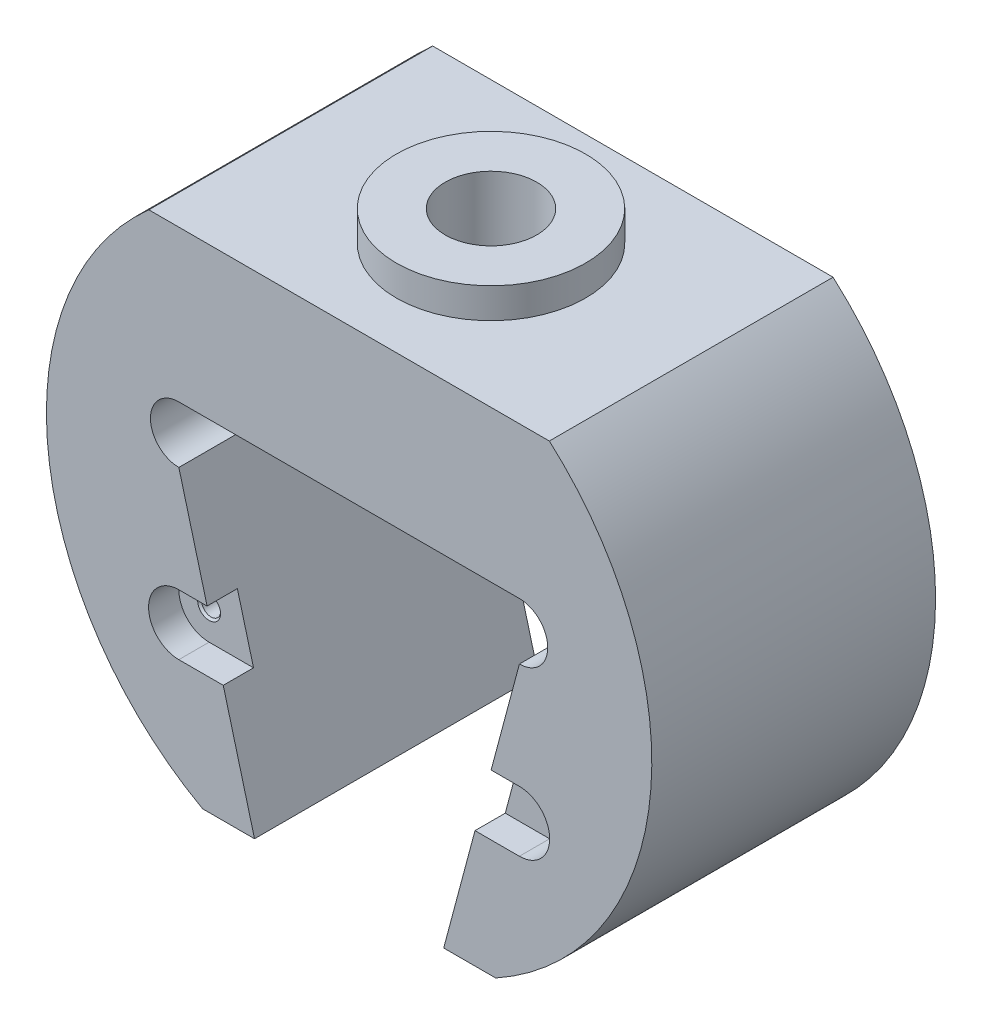
from build123d import *

# Parameters (mm, degrees)
SKETCH1_R                             = 80
BOSS_EXTRUDE1_DEPTH                   = 75
SKETCH2_OUTSIDE_W                     = 209.676
SKETCH2_OUTSIDE_H                     = 209.676
SKETCH2_OUTSIDE_W_2                   = 199.64377861
SKETCH2_OUTSIDE_H_2                   = 130
CUT_EXTRUDE1_DEPTH                    = 136.738719605
CUT_EXTRUDE2_DEPTH                    = 131.096118313
CUT_EXTRUDE3_DEPTH                    = 8
CUT_EXTRUDE4_START                    = -59
CUT_EXTRUDE4_DEPTH                    = 8
M6_TAPPED_HOLE1_D                     = 5
M6_TAPPED_HOLE1_DEPTH                 = 15
M6_TAPPED_HOLE1_CSINK_D               = 6.05
M6_TAPPED_HOLE1_CSINK_ANGLE           = 90
M6_TAPPED_HOLE1_TIP                   = 1.502151548
M6_TAPPED_HOLE1_ON_FACE_2_D           = 5
M6_TAPPED_HOLE1_ON_FACE_2_DEPTH       = 15
M6_TAPPED_HOLE1_ON_FACE_2_CSINK_D     = 6.05
M6_TAPPED_HOLE1_ON_FACE_2_CSINK_ANGLE = 90
M6_TAPPED_HOLE1_ON_FACE_2_TIP         = 1.502151548
CUT_EXTRUDE5_REACH                    = 172.074
SKETCH7_R                             = 12.1
BOSS_EXTRUDE4_START                   = 8
SKETCH8_R                             = 25
SKETCH8_R_2                           = 12.1
BOSS_EXTRUDE4_DEPTH                   = 8


with BuildPart() as part:
    # Sketch1 → Boss-Extrude1 (new body)
    with BuildSketch(Plane.XY):
        Circle(SKETCH1_R)
    extrude(amount=BOSS_EXTRUDE1_DEPTH)

    # Sketch2 outside → Cut-Extrude1 (cut, through all)
    with BuildSketch(Plane(origin=(0, 0, 0), x_dir=(-1, 0, 0), z_dir=(0, 0, -1))):
        Rectangle(SKETCH2_OUTSIDE_W, SKETCH2_OUTSIDE_H)
        with Locations((0.958801498, -5)):
            Rectangle(SKETCH2_OUTSIDE_W_2, SKETCH2_OUTSIDE_H_2, mode=Mode.SUBTRACT)
    extrude(amount=-CUT_EXTRUDE1_DEPTH, mode=Mode.SUBTRACT)

    # Sketch3 → Cut-Extrude2 (cut, through all)
    with BuildSketch(Plane(origin=(0, 0, 0), x_dir=(-1, 0, 0), z_dir=(0, 0, -1))):
        with BuildLine():
            Line((-25, -70), (-45, 5))
            ThreePointArc((-45, 5), (-52.5, 12.5), (-45, 20))
            Line((-45, 20), (45, 20))
            ThreePointArc((45, 20), (52.5, 12.5), (45, 5))
            Line((45, 5), (25, -70))
            Line((25, -70), (-25, -70))
        make_face()
    extrude(amount=-CUT_EXTRUDE2_DEPTH, mode=Mode.SUBTRACT)

    # Sketch4 → Cut-Extrude3 (cut)
    with BuildSketch(Plane(origin=(0, 0, 0), x_dir=(-1, 0, 0), z_dir=(0, 0, -1))):
        with BuildLine():
            Line((-45, -23), (45, -23))
            ThreePointArc((45, -23), (53, -31), (45, -39))
            Line((45, -39), (-45, -39))
            ThreePointArc((-45, -39), (-53, -31), (-45, -23))
        make_face()
    extrude(amount=-CUT_EXTRUDE3_DEPTH, mode=Mode.SUBTRACT)

    # Sketch5 → Cut-Extrude4 (cut)
    with BuildSketch(Plane(origin=(0, 0, 8), x_dir=(-1, 0, 0), z_dir=(0, 0, -1)).offset(CUT_EXTRUDE4_START)):
        with BuildLine():
            Line((37.533333333, -23), (33.266666667, -39))
            Line((33.266666667, -39), (45, -39))
            ThreePointArc((45, -39), (53, -31), (45, -23))
            Line((45, -23), (37.533333333, -23))
        make_face()
        with BuildLine():
            Line((-33.266666667, -39), (-37.533333333, -23))
            Line((-37.533333333, -23), (-45, -23))
            ThreePointArc((-45, -23), (-53, -31), (-45, -39))
            Line((-45, -39), (-33.266666667, -39))
        make_face()
    extrude(amount=-CUT_EXTRUDE4_DEPTH, mode=Mode.SUBTRACT)

    # M6 Tapped Hole1
    with Locations(Plane(origin=(45, -31, 8), x_dir=(-1, 0, 0), z_dir=(0, 0, -1))):
        with Locations((0, 0), (90, 0)):
            CounterSinkHole(M6_TAPPED_HOLE1_D / 2, M6_TAPPED_HOLE1_CSINK_D / 2, depth=M6_TAPPED_HOLE1_DEPTH, counter_sink_angle=M6_TAPPED_HOLE1_CSINK_ANGLE)
            with Locations((0, 0, -(M6_TAPPED_HOLE1_DEPTH + M6_TAPPED_HOLE1_TIP / 2))):  # 118° drill point
                Cone(0, M6_TAPPED_HOLE1_D / 2, M6_TAPPED_HOLE1_TIP, mode=Mode.SUBTRACT)

    # M6 Tapped Hole1 on face 2
    with Locations(Plane(origin=(-45, -31, 67), x_dir=(1, 0, 0), z_dir=(0, 0, 1))):
        with Locations((0, 0), (90, 0)):
            CounterSinkHole(M6_TAPPED_HOLE1_ON_FACE_2_D / 2, M6_TAPPED_HOLE1_ON_FACE_2_CSINK_D / 2, depth=M6_TAPPED_HOLE1_ON_FACE_2_DEPTH, counter_sink_angle=M6_TAPPED_HOLE1_ON_FACE_2_CSINK_ANGLE)
            with Locations((0, 0, -(M6_TAPPED_HOLE1_ON_FACE_2_DEPTH + M6_TAPPED_HOLE1_ON_FACE_2_TIP / 2))):  # 118° drill point
                Cone(0, M6_TAPPED_HOLE1_ON_FACE_2_D / 2, M6_TAPPED_HOLE1_ON_FACE_2_TIP, mode=Mode.SUBTRACT)

    # Sketch7 → Cut-Extrude5 (cut, up to next)
    with BuildSketch(Plane(origin=(0, 60, 0), x_dir=(1, 0, 0), z_dir=(0, 1, 0)), mode=Mode.PRIVATE) as cut_extrude5_sk1:
        with Locations(Location((0, -37.5, 0), (0, 0, 270))):
            Circle(SKETCH7_R)
    cut_extrude5_tool1 = extrude(cut_extrude5_sk1.sketch, amount=-CUT_EXTRUDE5_REACH, mode=Mode.PRIVATE) & part.part
    add(cut_extrude5_tool1.solids().sort_by_distance((0, 60, 37.5))[0], mode=Mode.SUBTRACT)

    # Sketch8 → Boss-Extrude4 (add)
    with BuildSketch(Plane(origin=(0, 60, 0), x_dir=(1, 0, 0), z_dir=(0, 1, 0)).offset(BOSS_EXTRUDE4_START)):
        with Locations(Location((0, -37.5, 0), (0, 0, 270))):
            Circle(SKETCH8_R)
        with Locations(Location((0, -37.5, 0), (0, 0, 270))):
            Circle(SKETCH8_R_2, mode=Mode.SUBTRACT)
    extrude(amount=-BOSS_EXTRUDE4_DEPTH)


solid = part.part
